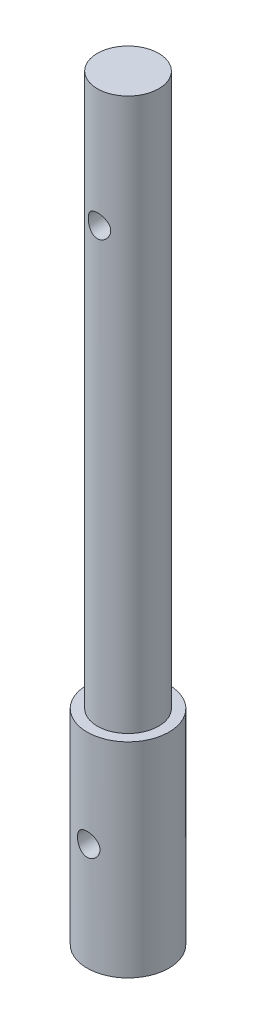
SolidWorks part; units mm, degrees
material "AISI 304"
ref_plane "前视基准面" through (0, 0, 0) normal (0, 0, 1) x (1, 0, 0)
ref_plane "上视基准面" through (0, 0, 0) normal (0, 1, 0) x (1, 0, 0)
ref_plane "右视基准面" through (0, 0, 0) normal (1, 0, 0) x (0, 0, -1)
sketch "草图1" plane through (0, 0, 0) normal (0, 0, 1) x (1, 0, 0)
  line L0 (0, 0) -> (0, 6982.6284) construction
  line L1 (0, 68.0974) -> (3, 68.0974)
  line L2 (3, 68.0974) -> (3, 14.0974)
  line L3 (3, 14.0974) -> (4, 14.0974)
  line L4 (4, 14.0974) -> (4, -5.9026)
  line L5 (4, -5.9026) -> (0, -5.9026)
  line L6 (0, 68.0974) -> (0, -5.9026)
  dimension "D1" = 3
  dimension "D2" = 4
  dimension "D3" = 74
  dimension "D4" = 54
revolve "旋转1" add sketch "草图1" angle 360 about L0
sketch "草图2" plane through (0, 0, 0) normal (0, 0, 1) x (1, 0, 0)
  line L0 (-4, -5.9026) -> (4, -5.9026) construction
  line L1 (3, 68.0974) -> (-3, 68.0974) construction
  line L2 (3, 14.0974) -> (3, 68.0974) construction
  line L3 (4, -5.9026) -> (4, 14.0974) construction
  circle A0 centre (0, 56.4974) radius 1.1
  circle A1 centre (0, 4.5974) radius 1.1
  dimension "D1" = 2.2
  dimension "D4" = 2.2
  dimension "D2" = 10.5
  dimension "D3" = 11.6
  dimension "D5" = 3
  dimension "D6" = 4
extrude "切除-拉伸1" cut sketch "草图2" against normal mid plane 30
